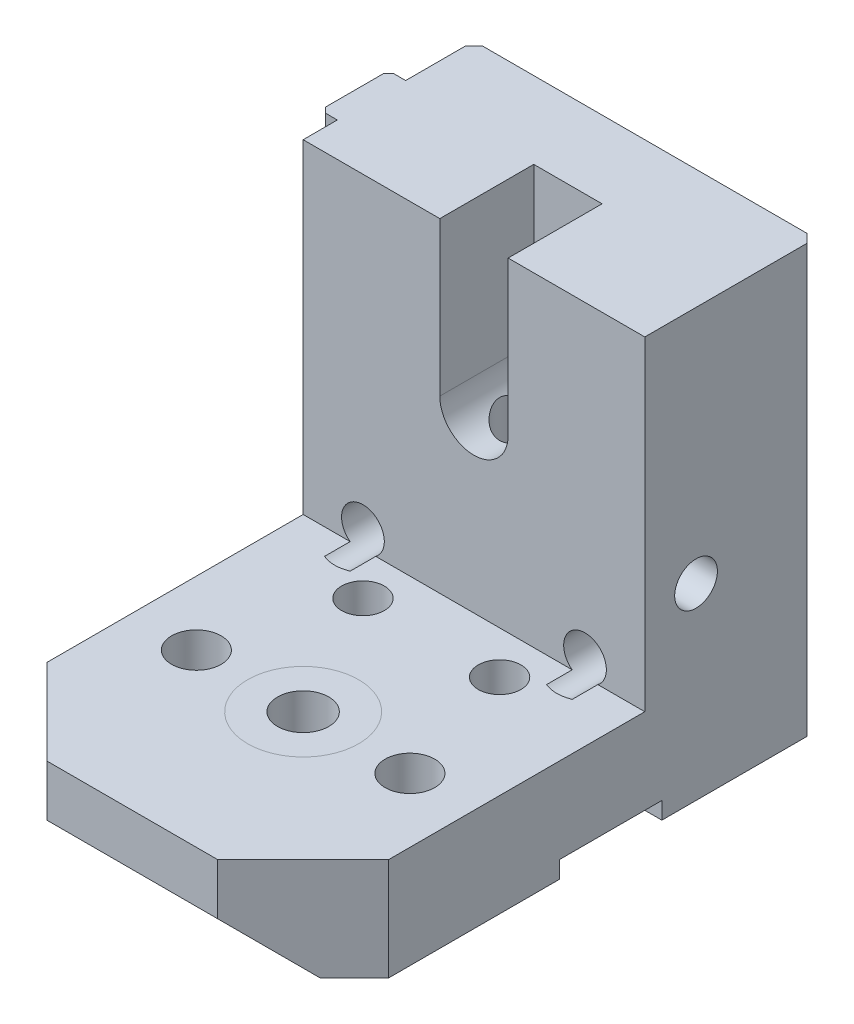
from build123d import *

# Parameters (mm, degrees)
SKETCH1_W                                   = 20
SKETCH1_H                                   = 25
BOSS_EXTRUDE1_DEPTH                         = 10
SKETCH2_W                                   = 20
SKETCH2_H                                   = 6
BOSS_EXTRUDE2_DEPTH                         = 20
SKETCH3_W                                   = 4
SKETCH3_H                                   = 11
CUT_EXTRUDE1_DEPTH                          = 9
SKETCH4_R                                   = 3.25
CUT_EXTRUDE2_DEPTH                          = 37.891733491
SKETCH5_R                                   = 3.25
SKETCH5_R_2                                 = 1.5
BOSS_EXTRUDE3_DEPTH                         = 6
HOLE_SIZE_PER_SOCKET_HEAD_CAP_SCREW_2_COUNT = 2
HOLE_SIZE_PER_SOCKET_HEAD_CAP_SCREW_2_PITCH = 12.5
SKETCH9_W                                   = 4
SKETCH9_H                                   = 25
BOSS_EXTRUDE4_DEPTH                         = 1
M3_TAPPED_HOLE1_AT_2_COUNT                  = 2
M3_TAPPED_HOLE1_AT_2_PITCH                  = 7
CHAMFER1_SIZE                               = 0.3
SKETCH13_R                                  = 2
CUT_EXTRUDE4_DEPTH                          = 5.5
M2_5_TAPPED_HOLE1_AT_2_COUNT                = 2
M2_5_TAPPED_HOLE1_AT_2_PITCH                = 16
CHAMFER2_SIZE                               = 5
CHAMFER3_SIZE                               = 0.5
M3_TAPPED_HOLE2_AT_2_COUNT                  = 2
M3_TAPPED_HOLE2_AT_2_PITCH                  = 13
M3_TAPPED_HOLE3_AT_2_COUNT                  = 2
M3_TAPPED_HOLE3_AT_2_PITCH                  = 8
SKETCH20_W                                  = 20
SKETCH20_H                                  = 6
CUT_EXTRUDE5_DEPTH                          = 1
CHAMFER4_SIZE                               = 3
SKETCH21_R                                  = 1.5
CUT_EXTRUDE9_DEPTH                          = 41.57092555


with BuildPart() as part:
    # Sketch1 → Boss-Extrude1 (new body)
    with BuildSketch(Plane.XY):
        Rectangle(SKETCH1_W, SKETCH1_H)
    extrude(amount=BOSS_EXTRUDE1_DEPTH)

    # Sketch2 → Boss-Extrude2 (add)
    with BuildSketch(Plane.XY.offset(10)):
        with Locations((0, -9.5)):
            Rectangle(SKETCH2_W, SKETCH2_H)
    extrude(amount=BOSS_EXTRUDE2_DEPTH)

    # Sketch3 → Cut-Extrude1 (cut)
    with BuildSketch(Plane(origin=(0, 12.5, 0), x_dir=(1, 0, 0), z_dir=(0, 1, 0))):
        with Locations((0, -10)):
            Rectangle(SKETCH3_W, SKETCH3_H)
    extrude(amount=-CUT_EXTRUDE1_DEPTH, mode=Mode.SUBTRACT)

    # Sketch4 → Cut-Extrude2 (cut, through all)
    with BuildSketch(Plane(origin=(0, -6.5, 0), x_dir=(1, 0, 0), z_dir=(0, 1, 0))):
        with Locations(Location((0, -20, 0), (0, 0, 270))):
            Circle(SKETCH4_R)
    extrude(amount=-CUT_EXTRUDE2_DEPTH, mode=Mode.SUBTRACT)

    # Sketch6 → Hole size per socket head cap screw type 1 (revolve, cut)
    with BuildSketch(Plane(origin=(6.25, -12.5, 20), x_dir=(0, 0, -1), z_dir=(1, 0, 0))):
        Polygon((0, 0), (0, 25.000025), (1.45, 25.000025), (1.45, 3.5), (2.5, 3.5), (2.5, 0), align=None)
    hole_size_per_socket_head_cap_screw_type = revolve(axis=Axis((6.25, -18.85, 20), (0, 1, 0)), mode=Mode.SUBTRACT)

    # Hole size per socket head cap screw  2: Hole size per socket head cap screw type 1 ×2
    with Locations(*[(-i * HOLE_SIZE_PER_SOCKET_HEAD_CAP_SCREW_2_PITCH, 0, 0) for i in range(1, HOLE_SIZE_PER_SOCKET_HEAD_CAP_SCREW_2_COUNT)]):
        add(hole_size_per_socket_head_cap_screw_type, mode=Mode.SUBTRACT)

    # Sketch9 → Boss-Extrude4 (add)
    with BuildSketch(Plane.ZY.offset(10)):
        with Locations((6, 0)):
            Rectangle(SKETCH9_W, SKETCH9_H)
    extrude(amount=BOSS_EXTRUDE4_DEPTH)

    # Sketch10 → M3 Tapped Hole1 (revolve, cut)
    with BuildSketch(Plane(origin=(-11, 5.5, 6), x_dir=(0, 0, 1), z_dir=(0, 1, 0))):
        Polygon((0, 0), (0, 8.251075774), (1.25, 7.5), (1.25, 0), align=None)
    m3_tapped_hole1 = revolve(axis=Axis((-17.35, 5.5, 6), (1, 0, 0)), mode=Mode.SUBTRACT)

    # M3 Tapped Hole1 at 2: M3 Tapped Hole1 ×2
    with Locations(*[(0, -i * M3_TAPPED_HOLE1_AT_2_PITCH, 0) for i in range(1, M3_TAPPED_HOLE1_AT_2_COUNT)]):
        add(m3_tapped_hole1, mode=Mode.SUBTRACT)

    # Chamfer1
    chamfer1_edges = [part.edges().sort_by_distance(p)[0] for p in [
        (-11, 0, 8),
        (-11, 0, 4),
    ]]
    chamfer(chamfer1_edges, length=CHAMFER1_SIZE)

    # Sketch13 → Cut-Extrude4 (cut)
    with BuildSketch(Plane.XY.offset(10)):
        with Locations((0, 3.5)):
            Circle(SKETCH13_R)
    extrude(amount=-CUT_EXTRUDE4_DEPTH, mode=Mode.SUBTRACT)

    # Sketch14 → M2.5 Tapped Hole1 (revolve, cut)
    with BuildSketch(Plane(origin=(8, 8.5, 0), x_dir=(0, 1, 0), z_dir=(1, 0, 0))):
        Polygon((0, 0), (0, 6.965882135), (1.025, 6.35), (1.025, 0), align=None)
    m2_5_tapped_hole1 = revolve(axis=Axis((8, 8.5, -6.35), (0, 0, 1)), mode=Mode.SUBTRACT)

    # M2.5 Tapped Hole1 at 2: M2.5 Tapped Hole1 ×2
    with Locations(*[(-i * M2_5_TAPPED_HOLE1_AT_2_PITCH, 0, 0) for i in range(1, M2_5_TAPPED_HOLE1_AT_2_COUNT)]):
        add(m2_5_tapped_hole1, mode=Mode.SUBTRACT)

    # Chamfer2
    chamfer2_edges = [part.edges().sort_by_distance(p)[0] for p in [
        (-10, -9.5, 30),
        (10, -9.5, 30),
    ]]
    chamfer(chamfer2_edges, length=CHAMFER2_SIZE)

    # Chamfer3
    chamfer3_edges = [part.edges().sort_by_distance(p)[0] for p in [
        (-10, 0, 0),
        (10, 0, 0),
    ]]
    chamfer(chamfer3_edges, length=CHAMFER3_SIZE)

    # Sketch16 → M3 Tapped Hole2 (revolve, cut)
    with BuildSketch(Plane(origin=(6.5, -5.5, 0), x_dir=(0, 1, 0), z_dir=(1, 0, 0))):
        Polygon((0, 0), (0, 12.251075774), (1.25, 11.5), (1.25, 0), align=None)
    m3_tapped_hole2 = revolve(axis=Axis((6.5, -5.5, -6.35), (0, 0, 1)), mode=Mode.SUBTRACT)

    # M3 Tapped Hole2 at 2: M3 Tapped Hole2 ×2
    with Locations(*[(-i * M3_TAPPED_HOLE2_AT_2_PITCH, 0, 0) for i in range(1, M3_TAPPED_HOLE2_AT_2_COUNT)]):
        add(m3_tapped_hole2, mode=Mode.SUBTRACT)

    # Sketch18 → M3 Tapped Hole3 (revolve, cut)
    with BuildSketch(Plane(origin=(-4, -12.5, 12.5), x_dir=(0, 0, -1), z_dir=(1, 0, 0))):
        Polygon((0, 0), (0, 8.251075774), (1.25, 7.5), (1.25, 0), align=None)
    m3_tapped_hole3 = revolve(axis=Axis((-4, -18.85, 12.5), (0, 1, 0)), mode=Mode.SUBTRACT)

    # M3 Tapped Hole3 at 2: M3 Tapped Hole3 ×2
    with Locations(*[(i * M3_TAPPED_HOLE3_AT_2_PITCH, 0, 0) for i in range(1, M3_TAPPED_HOLE3_AT_2_COUNT)]):
        add(m3_tapped_hole3, mode=Mode.SUBTRACT)

    # Sketch20 → Cut-Extrude5 (cut)
    with BuildSketch(Plane.XZ.offset(12.5)):
        with Locations((0, 12)):
            Rectangle(SKETCH20_W, SKETCH20_H)
    extrude(amount=-CUT_EXTRUDE5_DEPTH, mode=Mode.SUBTRACT)

    # Chamfer4
    chamfer4_edges = [part.edges().sort_by_distance(p)[0] for p in [
        (0, -12.5, 30),
    ]]
    chamfer(chamfer4_edges, length=CHAMFER4_SIZE)

    # Sketch21 → Cut-Extrude9 (cut, through all)
    with BuildSketch(Plane(origin=(0, 12.5, 0), x_dir=(1, 0, 0), z_dir=(0, 1, 0))):
        with Locations(Location((0, -7, 0), (0, 0, 270))):
            Circle(SKETCH21_R)
    extrude(amount=-CUT_EXTRUDE9_DEPTH, mode=Mode.SUBTRACT)

    # Sketch22 → M3 Tapped Hole4 (revolve, cut)
    with BuildSketch(Plane(origin=(10, -1.5, 7), x_dir=(0, 0, -1), z_dir=(0, 1, 0))):
        Polygon((0, 0), (0, 11.251075774), (1.25, 10.5), (1.25, 0), align=None)
    revolve(axis=Axis((16.35, -1.5, 7), (-1, 0, 0)), mode=Mode.SUBTRACT)


with BuildPart() as body_2:
    # Sketch5 → Boss-Extrude3 (new body)
    with BuildSketch(Plane(origin=(0, -6.5, 0), x_dir=(1, 0, 0), z_dir=(0, 1, 0))):
        with Locations(Location((0, -20, 0), (0, 0, 270))):
            Circle(SKETCH5_R)
        with Locations(Location((0, -20, 0), (0, 0, 270))):
            Circle(SKETCH5_R_2, mode=Mode.SUBTRACT)
    extrude(amount=-BOSS_EXTRUDE3_DEPTH)


solid = Compound([part.part, body_2.part])
